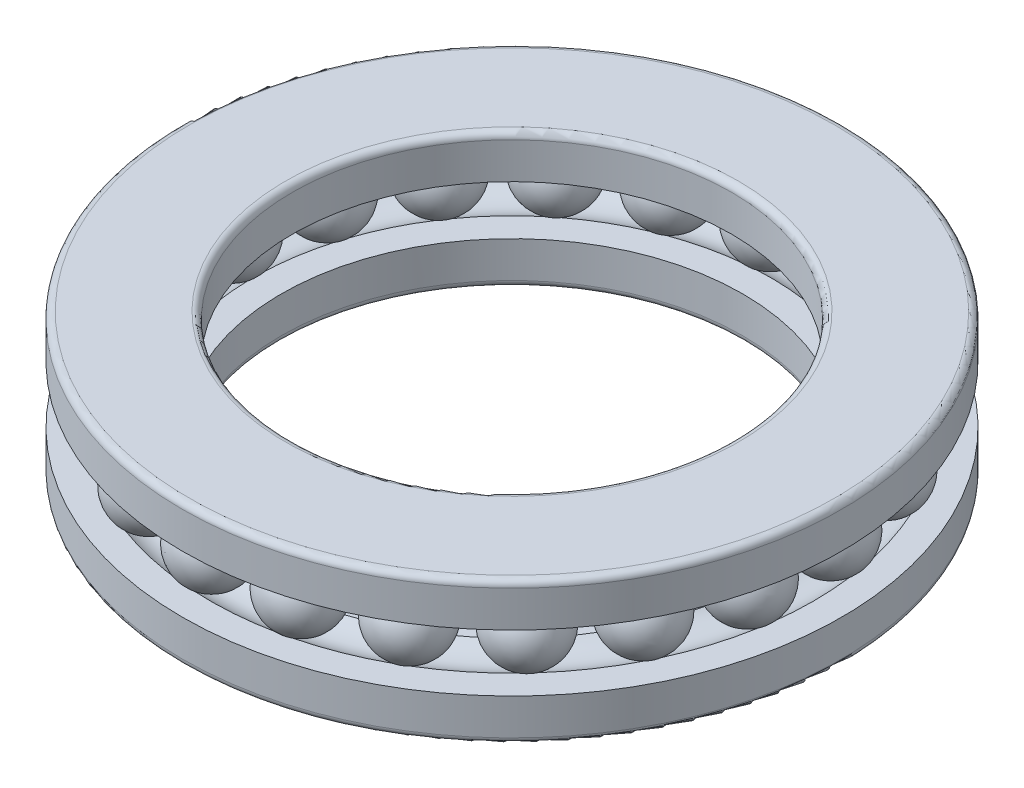
from build123d import *

# Parameters (mm, degrees)
CIRPATTERN1_COUNT = 21
FILLET1_R         = 0.6


with BuildPart() as part:
    # Sketch2 → Base-Revolve (revolve)
    with BuildSketch(Plane.XY, mode=Mode.PRIVATE) as base_revolve_sk:
        with BuildLine():
            Line((0, 3.9), (2.55, 3.9))
            ThreePointArc((2.55, 3.9), (4.5, 3.25), (6.45, 3.9))
            Line((6.45, 3.9), (9, 3.9))
            Line((9, 3.9), (9, 0))
            Line((9, 0), (0, 0))
            Line((0, 0), (0, 3.9))
        make_face()
    revolve(base_revolve_sk.sketch.rotate(Axis((30, 0, 0), (0, 1, 0)), 270), axis=Axis((30, 0, 0), (0, 1, 0)))

    # Sketch3 → Boss-Revolve2 (revolve)
    with BuildSketch(Plane.XY):
        with BuildLine():
            Line((4.5, 3.2), (4.5, 9.8))
            ThreePointArc((4.5, 9.8), (1.2, 6.5), (4.5, 3.2))
        make_face()
    boss_revolve2 = revolve(axis=Axis((4.5, 0, 0), (0, 1, 0)))

    # Sketch4 → Boss-Revolve3 (revolve)
    with BuildSketch(Plane.XY, mode=Mode.PRIVATE) as boss_revolve3_sk:
        with BuildLine():
            Line((0, 9.1), (2.55, 9.1))
            ThreePointArc((2.55, 9.1), (4.5, 9.75), (6.45, 9.1))
            Line((6.45, 9.1), (10, 9.1))
            Line((10, 9.1), (10, 13))
            Line((10, 13), (0, 13))
            Line((0, 13), (0, 9.1))
        make_face()
    revolve(boss_revolve3_sk.sketch.rotate(Axis((30, 0, 0), (0, 1, 0)), 270), axis=Axis((30, 0, 0), (0, 1, 0)))

    # CirPattern1: Boss-Revolve2 ×21 about axis
    cirpattern1_axis = Axis((30, 0, 0), (0, 1, 0))
    for i in range(1, CIRPATTERN1_COUNT):
        add(boss_revolve2.rotate(cirpattern1_axis, i * 360 / CIRPATTERN1_COUNT))

    # Fillet1
    fillet1_edges = [part.edges().sort_by_distance(p)[0] for p in [
        (30, 13, 20),
        (30, 13, 30),
        (30, 0, 21),
        (30, 0, 30),
    ]]
    fillet(fillet1_edges, radius=FILLET1_R)


solid = part.part
